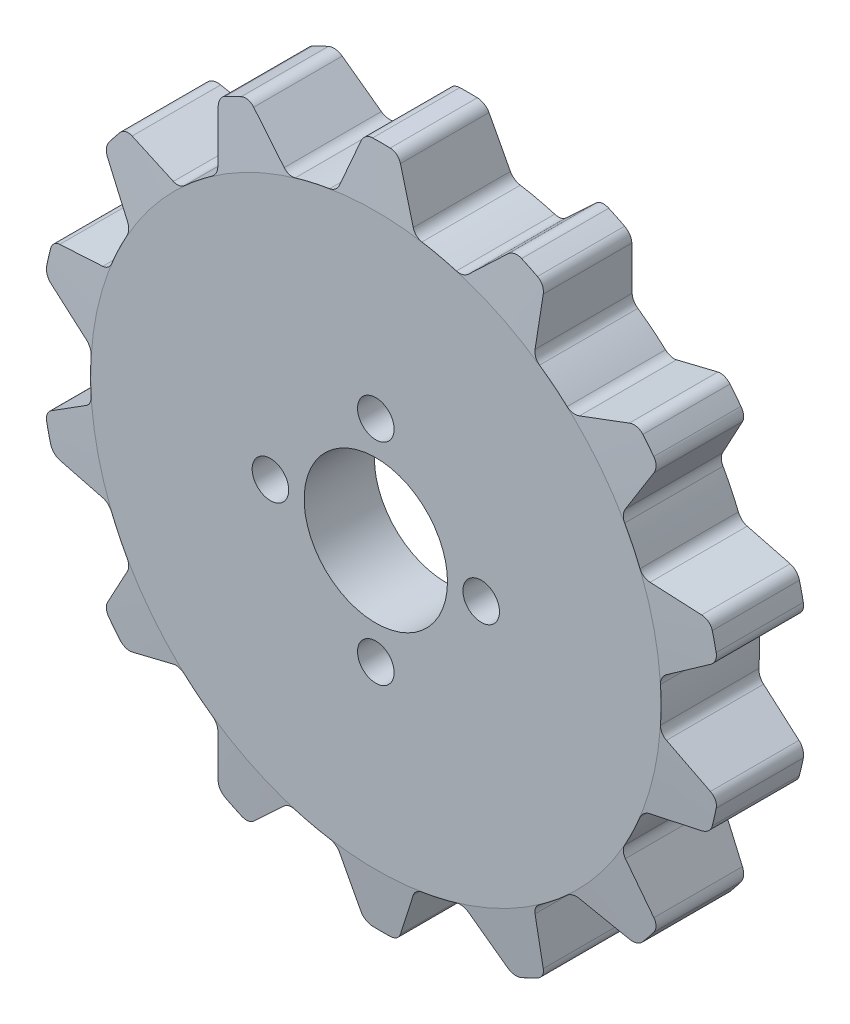
from build123d import *

# Parameters (mm, degrees)
SKETCH1_R           = 101.5
BOSS_EXTRUDE1_DEPTH = 35
BOSS_EXTRUDE2_START = -35
BOSS_EXTRUDE2_DEPTH = 35
CIRPATTERN1_COUNT   = 14
SKETCH4_R           = 25.5
CUT_EXTRUDE1_DEPTH  = 174.765991004
SKETCH8_R           = 6.5
CUT_EXTRUDE2_DEPTH  = 174.765991004
SKETCH9_R           = 50.5
CUT_EXTRUDE3_DEPTH  = 10


with BuildPart() as part:
    # Sketch1 → Boss-Extrude1 (new body)
    with BuildSketch(Plane.XY):
        Circle(SKETCH1_R)
    extrude(amount=BOSS_EXTRUDE1_DEPTH)

    # Sketch2 → Boss-Extrude2 (add)
    with BuildSketch(Plane.XY.offset(35).offset(BOSS_EXTRUDE2_START)):
        with BuildLine():
            Line((-7.012482665, 118.716532908), (-13.107442453, 102.852940998))
            ThreePointArc((-13.107442453, 102.852940998), (-14.400719403, 101.068769566), (-16.41028632, 100.164627004))
            ThreePointArc((-16.41028632, 100.164627004), (0, 101.5), (16.41028632, 100.164627004))
            ThreePointArc((16.41028632, 100.164627004), (14.400719403, 101.068769566), (13.107442453, 102.852940998))
            Line((13.107442453, 102.852940998), (7.012482665, 118.716532908))
            ThreePointArc((7.012482665, 118.716532908), (5.486320427, 120.67738563), (3.127920292, 121.459730424))
            ThreePointArc((3.127920292, 121.459730424), (0, 121.5), (-3.127920292, 121.459730424))
            ThreePointArc((-3.127920292, 121.459730424), (-5.486320427, 120.67738563), (-7.012482665, 118.716532908))
        make_face()
    boss_extrude2 = extrude(amount=BOSS_EXTRUDE2_DEPTH)

    # CirPattern1: Boss-Extrude2 ×14 about axis
    cirpattern1_axis = Axis((0, 0, 0), (0, 0, 1))
    for i in range(1, CIRPATTERN1_COUNT):
        add(boss_extrude2.rotate(cirpattern1_axis, i * 360 / CIRPATTERN1_COUNT))

    # Sketch3 → Cut-Revolve1 (revolve, cut)
    with BuildSketch(Plane(origin=(0, 0, 0), x_dir=(0, 0, -1), z_dir=(1, 0, 0)), mode=Mode.PRIVATE) as cut_revolve1_sk:
        Polygon((-35, 121.459730424), (-35, 101.459730424), (-33, 121.459730424), (-33, 126.15998601), (-35, 126.15998601), align=None)
        Polygon((0, 126.15998601), (0, 121.459730424), (0, 101.459730424), (-2, 121.459730424), (-2, 126.15998601), align=None)
    revolve(cut_revolve1_sk.sketch.rotate(Axis((0, 0, 35), (0, 0, -1)), 273.552853633), axis=Axis((0, 0, 35), (0, 0, -1)), mode=Mode.SUBTRACT)

    # Sketch4 → Cut-Extrude1 (cut, through all)
    with BuildSketch(Plane.XY.offset(35)):
        Circle(SKETCH4_R)
    extrude(amount=-CUT_EXTRUDE1_DEPTH, mode=Mode.SUBTRACT)

    # Sketch8 → Cut-Extrude2 (cut, through all)
    with BuildSketch(Plane(origin=(0, 0, 0), x_dir=(-1, 0, 0), z_dir=(0, 0, -1))):
        with Locations((0, 37.5)):
            Circle(SKETCH8_R)
        with Locations((37.5, 0)):
            Circle(SKETCH8_R)
        with Locations((0, -37.5)):
            Circle(SKETCH8_R)
        with Locations((-37.5, 0)):
            Circle(SKETCH8_R)
    extrude(amount=-CUT_EXTRUDE2_DEPTH, mode=Mode.SUBTRACT)

    # Sketch9 → Cut-Extrude3 (cut)
    with BuildSketch(Plane(origin=(0, 0, 0), x_dir=(-1, 0, 0), z_dir=(0, 0, -1))):
        Circle(SKETCH9_R)
    extrude(amount=-CUT_EXTRUDE3_DEPTH, mode=Mode.SUBTRACT)


solid = part.part
